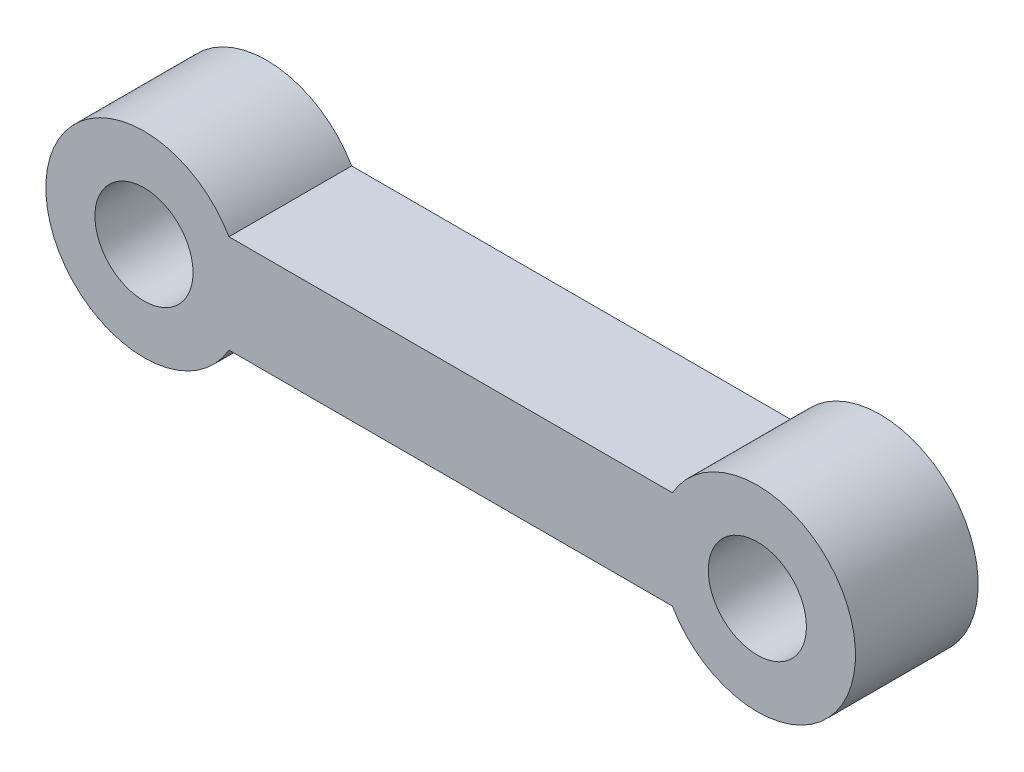
SolidWorks part; units mm, degrees
ref_plane "Front Plane" through (0, 0, 0) normal (0, 0, 1) x (1, 0, 0)
ref_plane "Top Plane" through (0, 0, 0) normal (0, 1, 0) x (1, 0, 0)
ref_plane "Right Plane" through (0, 0, 0) normal (1, 0, 0) x (0, 0, -1)
sketch "Sketch1" plane through (0, 0, 0) normal (0, 0, 1) x (1, 0, 0)
  line L0 (6.9282, -4) -> (43.0718, -4)
  line L1 (6.9282, 4) -> (43.0718, 4)
  line L2 (0, 0) -> (50, 0) construction
  circle A0 centre (0, 0) radius 4
  arc A1 (6.9282, 4) -> (6.9282, -4) centre (0, 0) ccw
  circle A2 centre (50, 0) radius 4
  arc A3 (43.0718, -4) -> (43.0718, 4) centre (50, 0) ccw
  dimension "D1" = 50
  dimension "D2" = 8
  dimension "D3" = 8
  dimension "D4" = 16
  dimension "D5" = 16
  dimension "D6" = 8
  dimension "D7" = 4
extrude "Boss-Extrude1" add sketch "Sketch1" along normal blind 10
